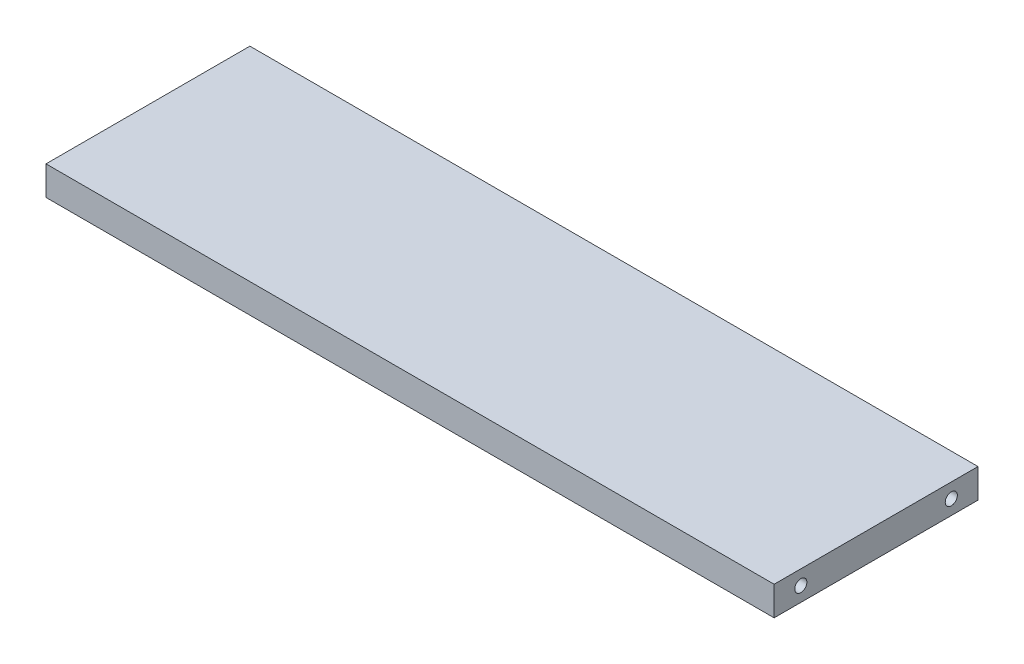
SolidWorks part; units mm, degrees
material "Q235B"
ref_plane "Front Plane" through (0, 0, 0) normal (0, 0, 1) x (1, 0, 0)
ref_plane "Top Plane" through (0, 0, 0) normal (0, 1, 0) x (1, 0, 0)
ref_plane "Right Plane" through (0, 0, 0) normal (1, 0, 0) x (0, 0, -1)
sketch "Sketch1" plane through (0, 0, 0) normal (0, 1, 0) x (1, 0, 0)
  line L1 (-75, 21) -> (75, 21)
  line L2 (-75, 21) -> (-75, -21)
  line L3 (-75, -21) -> (75, -21)
  line L4 (75, 21) -> (75, -21)
  line L5 (-75, 21) -> (75, -21) construction
  line L6 (-75, -21) -> (75, 21) construction
  point P0 (0, 0)
  dimension "D1" = 42
  dimension "D2" = 150
extrude "Boss-Extrude1" add sketch "Sketch1" along normal blind 6
sketch "Sketch2" plane through (75, 0, 0) normal (1, 0, 0) x (0, 0, -1)
  line L1 (-21, 0) -> (21, 0) construction
  line L2 (-21, 6) -> (-21, 0) construction
  circle A0 centre (15.5, 3) radius 1.25
  circle A1 centre (-15.5, 3) radius 1.25
  dimension "D1" = 2.5
  dimension "D2" = 3
  dimension "D3" = 31
  dimension "D4" = 5.5
extrude "Cut-Extrude1" cut sketch "Sketch2" against normal blind 5
cosmetic thread "HoleThreadLine1" parameters "D1"=6, "D2"=3
cosmetic thread "HoleThreadLine2" parameters "D1"=6, "D2"=3
sketch "Sketch3" plane through (-75, 0, 0) normal (-1, 0, 0) x (0, 0, 1)
  line L0 (-21, 0) -> (21, 0) construction
  line L1 (-21, 6) -> (-21, 0) construction
  circle A0 centre (-15.5, 3) radius 1.25
  circle A1 centre (15.5, 3) radius 1.25
  dimension "D1" = 2.5
  dimension "D2" = 3
  dimension "D3" = 31
  dimension "D4" = 5.5
extrude "Cut-Extrude2" cut sketch "Sketch3" against normal blind 5
cosmetic thread "HoleThreadLine3" parameters "D1"=6, "D2"=3
cosmetic thread "HoleThreadLine4" parameters "D1"=6, "D2"=3
hole_wizard "M3 Tapped Hole1" positions "Sketch4" profile "Sketch5" tap size "M3" standard "GB"
sketch "Sketch4" plane through (75, 0, 0) normal (1, 0, 0) x (0, 0, -1)
  point P0 (-15.5, 3)
  point P3 (15.5, 3)
sketch "Sketch5" plane through (75, 3, 15.5) normal (0, 1, 0) x (0, 0, -1)
  line L0 (0, 0) -> (0, 8.2511)
  line L1 (0, 8.2511) -> (1.25, 7.5)
  line L2 (1.25, 7.5) -> (1.25, 0)
  line L5 (1.25, 0) -> (0, 0)
  line L10 (0, 8.2511) -> (-1.25, 7.5) construction
  line L11 (0, -6.35) -> (0, 107.95) construction
  dimension "螺纹孔钻头直径" = 2.5
  dimension "螺纹孔钻头深度" = 7.5
  dimension "导头角度" = 118
hole_wizard "M3 Tapped Hole2" positions "Sketch6" profile "Sketch7" tap size "M3" standard "GB"
sketch "Sketch6" plane through (-75, 0, 0) normal (-1, 0, 0) x (0, 0, 1)
  point P0 (-15.5, 3)
  point P3 (15.5, 3)
sketch "Sketch7" plane through (-75, 3, -15.5) normal (0, 1, 0) x (0, 0, 1)
  line L0 (0, 0) -> (0, 8.2511)
  line L1 (0, 8.2511) -> (1.25, 7.5)
  line L2 (1.25, 7.5) -> (1.25, 0)
  line L5 (1.25, 0) -> (0, 0)
  line L10 (0, 8.2511) -> (-1.25, 7.5) construction
  line L11 (0, -6.35) -> (0, 107.95) construction
  dimension "螺纹孔钻头直径" = 2.5
  dimension "螺纹孔钻头深度" = 7.5
  dimension "导头角度" = 118
